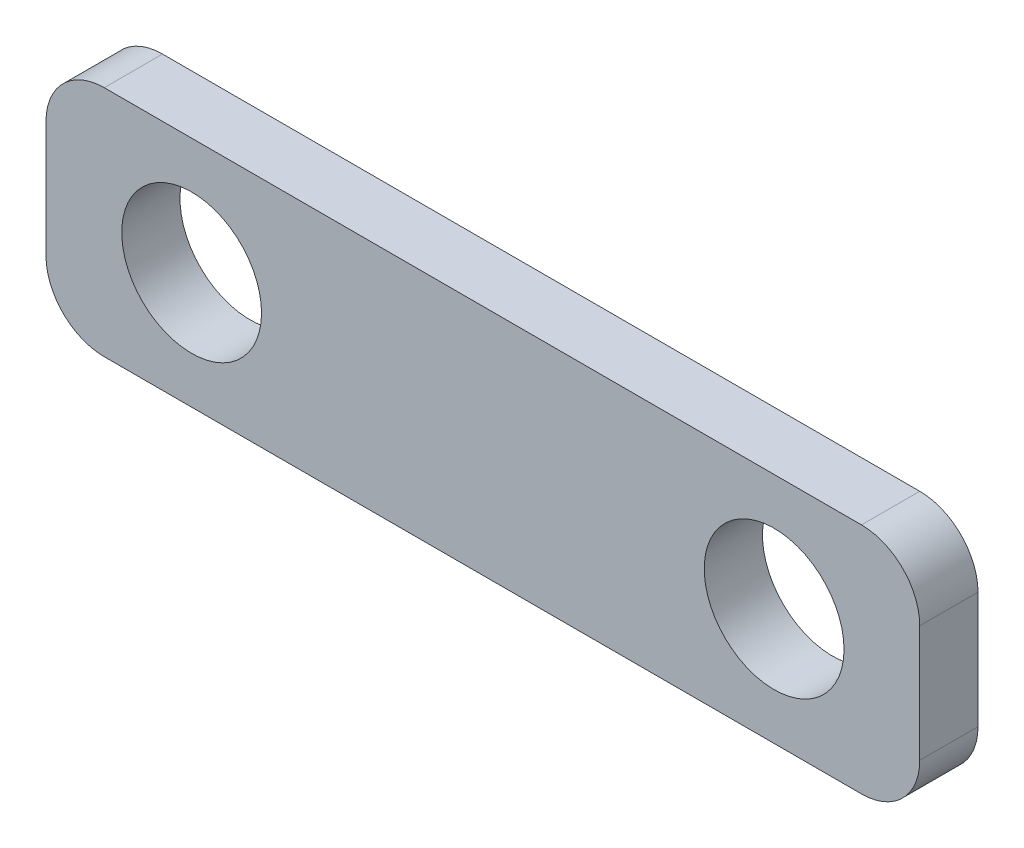
SolidWorks part; units mm, degrees
ref_plane "Front Plane" through (0, 0, 0) normal (0, 0, 1) x (1, 0, 0)
ref_plane "Top Plane" through (0, 0, 0) normal (0, 1, 0) x (1, 0, 0)
ref_plane "Right Plane" through (0, 0, 0) normal (1, 0, 0) x (0, 0, -1)
other "Configuration Table"
sketch "Sketch1" plane through (0, 0, 0) normal (0, 0, 1) x (1, 0, 0)
  line L1 (-75, 20) -> (75, 20)
  line L2 (-75, 20) -> (-75, -20)
  line L3 (-75, -20) -> (75, -20)
  line L4 (75, 20) -> (75, -20)
  line L5 (-75, 20) -> (75, -20) construction
  line L6 (-75, -20) -> (75, 20) construction
  circle A0 centre (50, 0) radius 12
  circle A1 centre (-50, 0) radius 12
  point P0 (0, 0)
  dimension "D3" = 24
  dimension "D4" = 24
  dimension "D5" = 25
  dimension "D1" = 150
  dimension "D2" = 40
  dimension "D6" = 25
extrude "Boss-Extrude1" add sketch "Sketch1" along normal blind 10
fillet "Fillet1" radius 10 4 edges at (75, 20, 5) (-75, -20, 5) (-75, 20, 5) (75, -20, 5)
